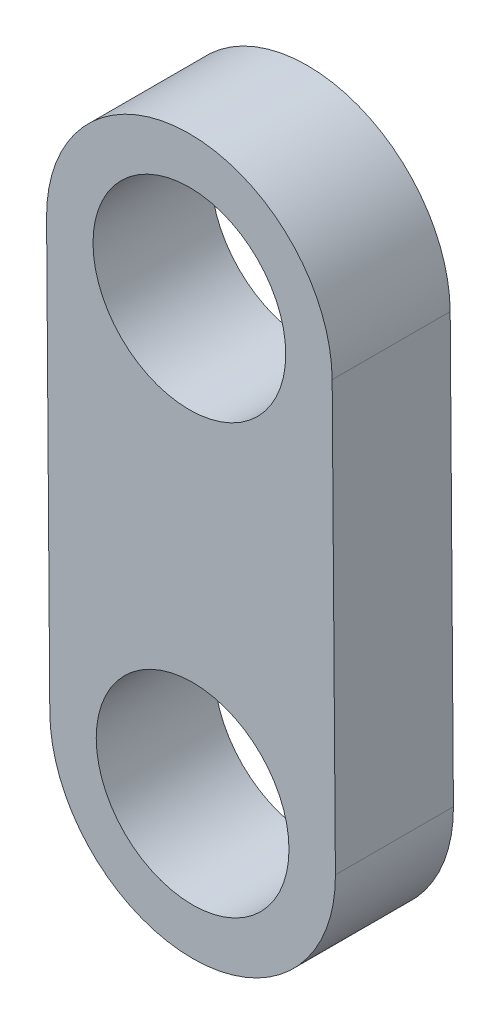
from build123d import *

# Parameters (mm, degrees)
SKETCH1_R           = 3.674588618
BOSS_EXTRUDE1_DEPTH = 4.5


with BuildPart() as part:
    # Sketch1 → Boss-Extrude1 (new body)
    with BuildSketch(Plane.XY):
        with BuildLine():
            Line((31.69623991, -16.220097286), (31.57303389, 0.068183186))
            ThreePointArc((31.57303389, 0.068183186), (26.087023529, 5.47182325), (20.683383464, -0.014187111))
            Line((20.683383464, -0.014187111), (20.806589485, -16.302467582))
            ThreePointArc((20.806589485, -16.302467582), (26.292599845, -21.706107647), (31.69623991, -16.220097286))
        make_face()
        with Locations((26.128208677, 0.026998038)):
            Circle(SKETCH1_R, mode=Mode.SUBTRACT)
        with Locations((26.251414697, -16.261282434)):
            Circle(SKETCH1_R, mode=Mode.SUBTRACT)
    extrude(amount=BOSS_EXTRUDE1_DEPTH)


solid = part.part
